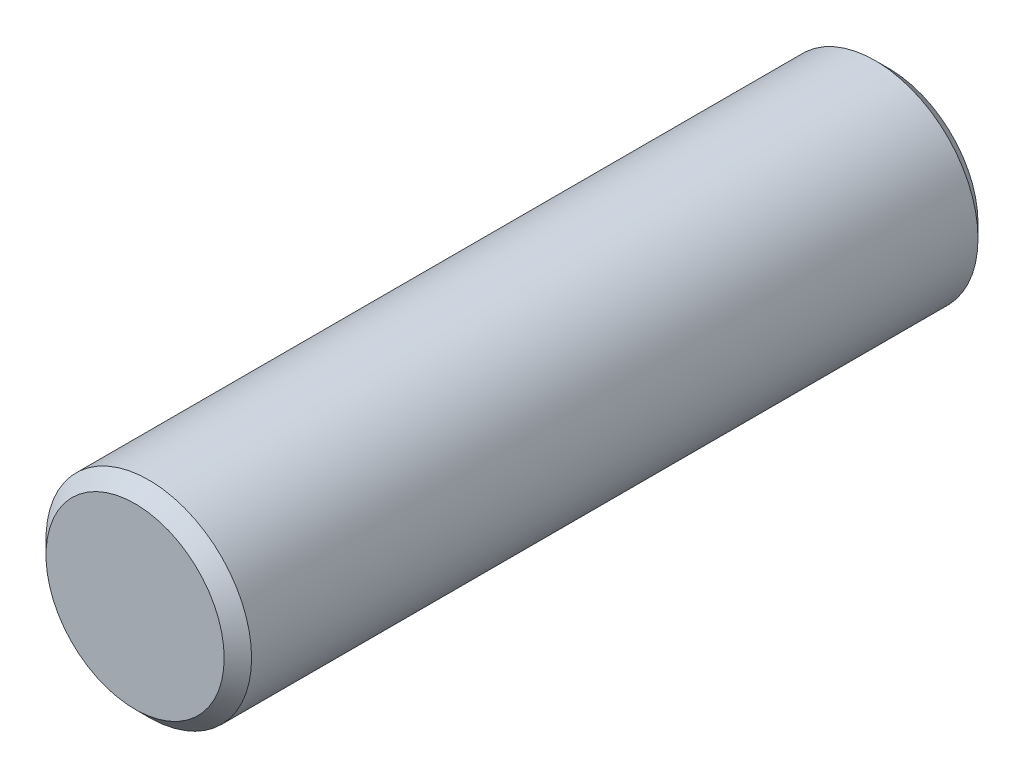
SolidWorks part; units mm, degrees
ref_plane "Front Plane" through (0, 0, 0) normal (0, 0, 1) x (1, 0, 0)
ref_plane "Top Plane" through (0, 0, 0) normal (0, 1, 0) x (1, 0, 0)
ref_plane "Right Plane" through (0, 0, 0) normal (1, 0, 0) x (0, 0, -1)
sketch "Sketch1" plane through (0, 0, 0) normal (0, 0, 1) x (1, 0, 0)
  circle A0 centre (0, 8.5691) radius 1.5 construction
  circle A1 centre (0, 8.5691) radius 1.5
extrude "Boss-Extrude1" add sketch "Sketch1" against normal blind 11
chamfer "Chamfer1" distance 0.2 angle 45 2 edges at (1.5, 8.5691, 0) (1.5, 8.5691, -11)
